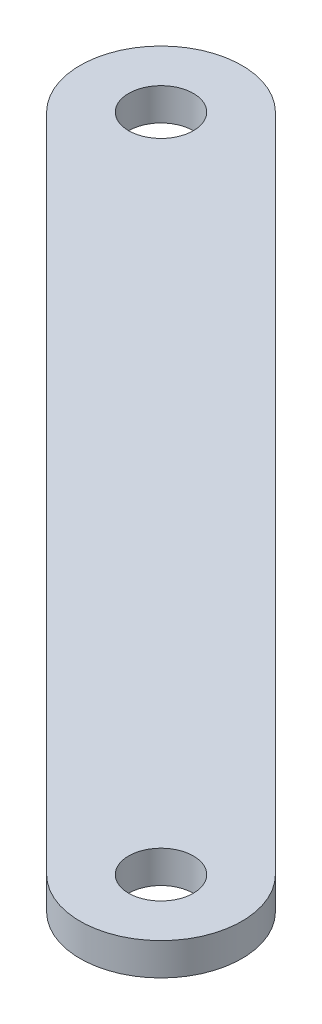
SolidWorks part; units mm, degrees
ref_plane "Plan de face" through (0, 0, 0) normal (0, 0, 1) x (1, 0, 0)
ref_plane "Plan de dessus" through (0, 0, 0) normal (0, 1, 0) x (1, 0, 0)
ref_plane "Plan de droite" through (0, 0, 0) normal (1, 0, 0) x (0, 0, -1)
sketch "Sketch1" plane through (0, 0, 0) normal (0, 1, 0) x (1, 0, 0)
  line L0 (45.1652, -40.8175) -> (-36.4698, 40.8175) construction
  line L1 (38.0941, -47.8885) -> (-43.5409, 33.7464)
  line L2 (52.2362, -33.7464) -> (-29.3987, 47.8885)
  line L3 (1.2442, -42.1743) -> (-4.3181, -41.1439) construction
  line L4 (-4.3181, -41.1439) -> (-55.1652, 32.827) construction
  line L5 (-55.1652, 32.827) -> (-36.4698, 40.8175) construction
  arc A0 (38.0941, -47.8885) -> (52.2362, -33.7464) centre (45.1652, -40.8175) ccw
  arc A1 (-29.3987, 47.8885) -> (-43.5409, 33.7464) centre (-36.4698, 40.8175) ccw
  circle A2 centre (45.1652, -40.8175) radius 4
  circle A3 centre (-36.4698, 40.8175) radius 4
  point P2 (4.3477, 0)
extrude "Boss.-Extru.1" add sketch "Sketch1" along normal blind 4
